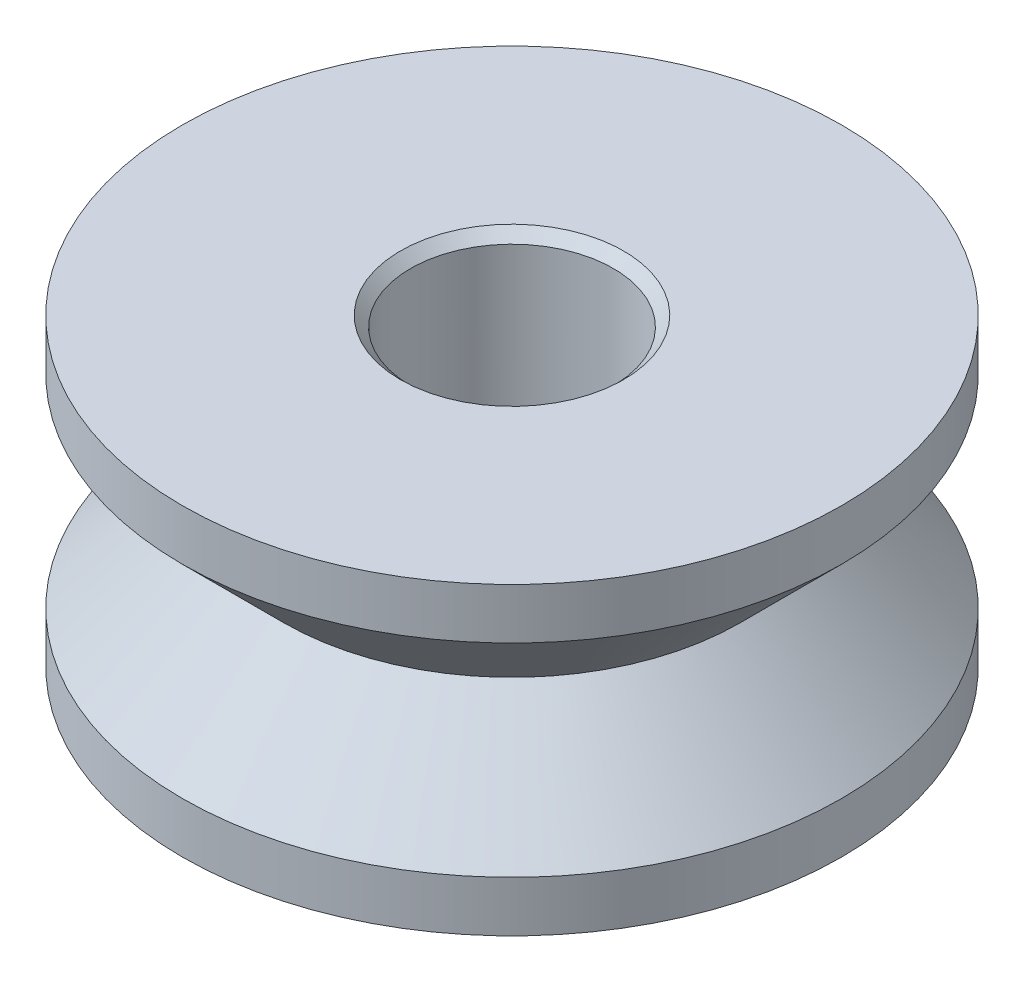
from build123d import *

# Parameters (mm, degrees)
SKETCH_1_R          = 4.5
SKETCH_2_R          = 6.5
SKETCH_3_R          = 6.5
EXTRUDE_1_DEPTH     = 1
SKETCH_4_R          = 2
CUT_EXTRUDE_1_DEPTH = 11.977249318
CHAMFER_1_SIZE      = 0.2


with BuildPart() as part:
    # 草图1 → 放样1 section 0
    with BuildSketch(Plane(origin=(0, 0, 0), x_dir=(1, 0, 0), z_dir=(0, 1, 0))):
        Circle(SKETCH_1_R)
    # 草图2 → 放样1 section 1
    with BuildSketch(Plane(origin=(0, 2, 0), x_dir=(1, 0, 0), z_dir=(0, 1, 0))):
        Circle(SKETCH_2_R)
    loft_1 = loft()

    # 草图3 → 凸台-拉伸1 (add)
    with BuildSketch(Plane(origin=(0, 2, 0), x_dir=(1, 0, 0), z_dir=(0, 1, 0))):
        with Locations(Location((0, 0, 0), (0, 0, 270))):
            Circle(SKETCH_3_R)
    extrude_1 = extrude(amount=EXTRUDE_1_DEPTH)

    # 镜向1: 放样1, 凸台-拉伸1 across plane
    add(loft_1.mirror(Plane.ZX))
    add(extrude_1.mirror(Plane.ZX))

    # 草图4 → 切除-拉伸1 (cut, through all)
    with BuildSketch(Plane(origin=(0, 3, 0), x_dir=(1, 0, 0), z_dir=(0, 1, 0))):
        with Locations(Location((0, 0, 0), (0, 0, 270))):
            Circle(SKETCH_4_R)
    extrude(amount=-CUT_EXTRUDE_1_DEPTH, mode=Mode.SUBTRACT)

    # 倒角1
    chamfer_1_edges = [part.edges().sort_by_distance(p)[0] for p in [
        (0, -3, -2),
        (0, 3, -2),
    ]]
    chamfer(chamfer_1_edges, length=CHAMFER_1_SIZE)


solid = part.part
